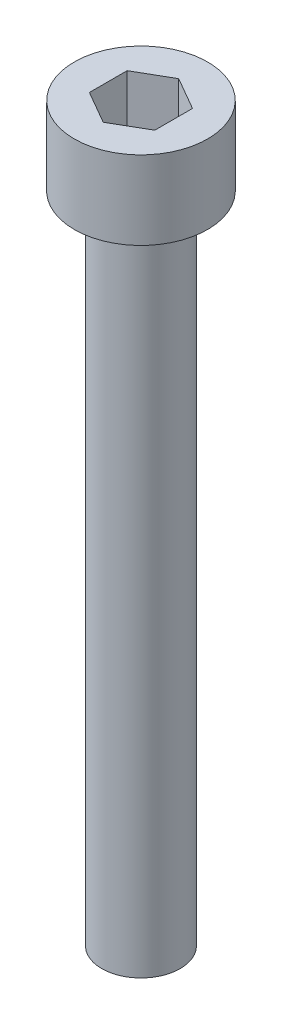
SolidWorks part; units mm, degrees
ref_plane "Front Plane" through (0, 0, 0) normal (0, 0, 1) x (1, 0, 0)
ref_plane "Top Plane" through (0, 0, 0) normal (0, 1, 0) x (1, 0, 0)
ref_plane "Right Plane" through (0, 0, 0) normal (1, 0, 0) x (0, 0, -1)
sketch "Sketch 1" plane through (0, 0, 0) normal (0, 0, 1) x (1, 0, 0)
  line L0 (0, 11.322) -> (0, -25.8305) construction
  line L1 (-9.8983, 0) -> (13.1525, 0) construction
  line L2 (0, 6) -> (-5.1, 6)
  line L3 (-5.1, 6) -> (-5.1, 0)
  line L4 (-5.1, 0) -> (-3, 0)
  line L5 (-3, 0) -> (-3, -50)
  line L6 (-3, -50) -> (0, -50)
  line L7 (0, -50) -> (0, 6)
  dimension "D1" = 6
  dimension "D2" = 50
  dimension "D3" = 6
  dimension "D4" = 10.2
revolve "Revolve 1" add sketch "Sketch 1" angle 360 about L0
sketch "Sketch 2" plane through (0, 6, 0) normal (0, 1, 0) x (1, 0, 0)
  line L1 (0, 2.8868) -> (-2.5, 1.4434)
  line L2 (-2.5, 1.4434) -> (-2.5, -1.4434)
  line L3 (-2.5, -1.4434) -> (0, -2.8868)
  line L4 (0, -2.8868) -> (2.5, -1.4434)
  line L5 (2.5, -1.4434) -> (2.5, 1.4434)
  line L6 (2.5, 1.4434) -> (0, 2.8868)
  circle A0 centre (0, 0) radius 2.5 construction
  dimension "D1" = 5
extrude "Cut-Extrude 1" cut sketch "Sketch 2" against normal blind 5
